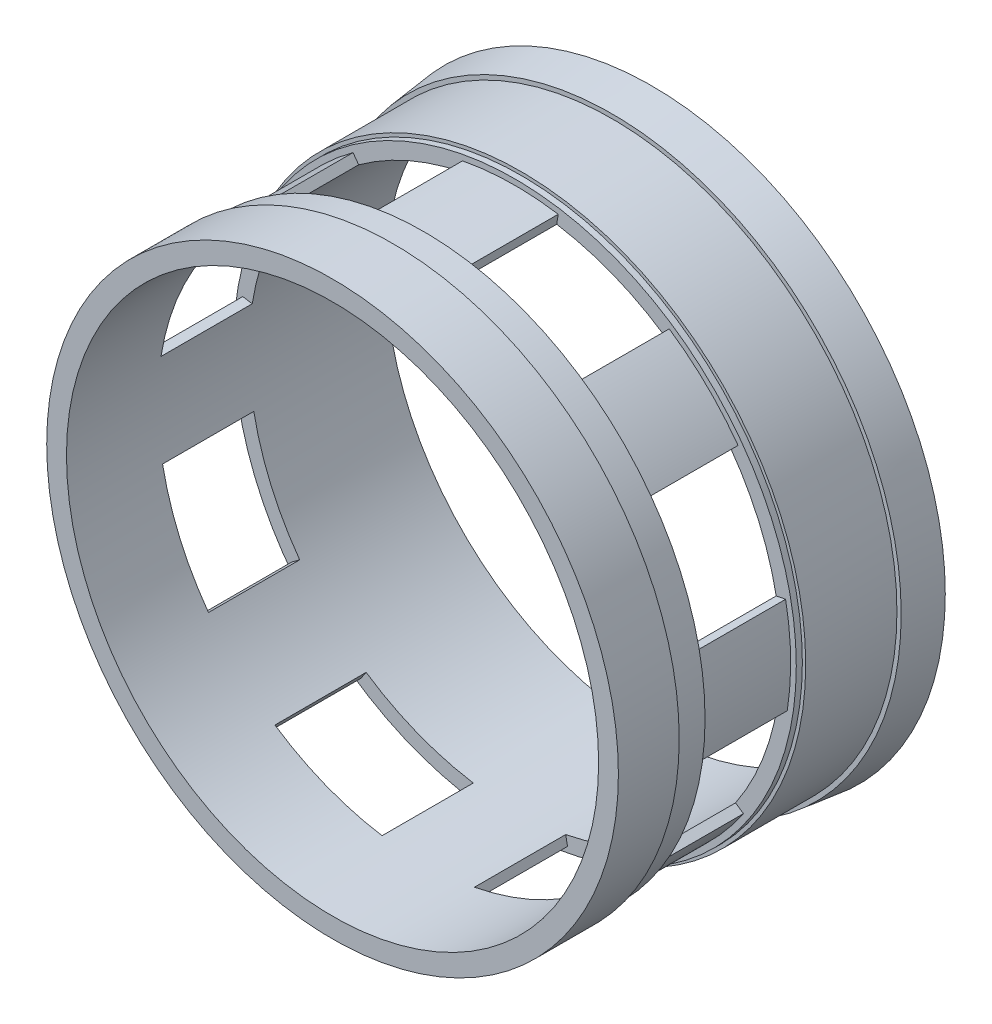
SolidWorks part; units mm, degrees
ref_plane "Front Plane" through (0, 0, 0) normal (0, 0, 1) x (1, 0, 0)
ref_plane "Top Plane" through (0, 0, 0) normal (0, 1, 0) x (1, 0, 0)
ref_plane "Right Plane" through (0, 0, 0) normal (1, 0, 0) x (0, 0, -1)
sketch "Sketch1" plane through (0, 0, 0) normal (0, 0, 1) x (1, 0, 0)
  circle A0 centre (0, 0) radius 9.65
  dimension "D1" = 19.3
ref_plane "Plane1" through (0, 0, 1.3) normal (0, 0, 1) x (1, 0, 0)
sketch "Sketch2" plane through (0, 0, 1.3) normal (0, 0, 1) x (1, 0, 0)
  circle A0 centre (0, 0) radius 9.5
  dimension "D1" = 19
loft "Loft2" add profiles "Sketch1", "Sketch2"
sketch "Sketch3" plane through (0, 0, 1.3) normal (0, 0, 1) x (1, 0, 0)
  circle A0 centre (0, 0) radius 9.36
  dimension "D1" = 18.72
extrude "Boss-Extrude1" add sketch "Sketch3" along normal blind 3
sketch "Sketch4" plane through (0, 0, 4.3) normal (0, 0, 1) x (1, 0, 0)
  circle A0 centre (0, 0) radius 9.25
  dimension "D1" = 18.5
extrude "Boss-Extrude2" add sketch "Sketch4" along normal blind 0.2
sketch "Sketch5" plane through (0, 0, 4.5) normal (0, 0, 1) x (1, 0, 0)
  circle A0 centre (0, 0) radius 8.75
  dimension "D1" = 17.5
extrude "Cut-Extrude1" cut sketch "Sketch5" against normal blind 10.2
sketch "Sketch7" plane through (0, 0, 4.5) normal (0, 0, 1) x (1, 0, 0)
  line L0 (-1.6668, 8.5898) -> (-1.7268, 8.8989)
  line L1 (0, 0) -> (-0.1765, 10.3009) construction
  line L2 (1.3716, 8.6418) -> (1.4209, 8.9528)
  arc A0 (1.3716, 8.6418) -> (-1.6668, 8.5898) centre (0, 0) ccw
  arc A1 (1.4209, 8.9528) -> (-1.7268, 8.8989) centre (0, 0) ccw
  dimension "D1" = 10
extrude "Boss-Extrude3" add sketch "Sketch7" along normal blind 3
pattern_circular "CirPattern1" count 8 over 360 about axis through (0, 0, 0) along (0, 0, 1) of "Boss-Extrude3"
sketch "Sketch8" plane through (0, 0, 7.5) normal (0, 0, 1) x (1, 0, 0)
  circle A0 centre (0, 0) radius 9.25
extrude "Boss-Extrude4" add sketch "Sketch8" along normal blind 1
sketch "Sketch9" plane through (0, 0, 8.5) normal (0, 0, 1) x (1, 0, 0)
  circle A0 centre (0, 0) radius 9.4
  dimension "D1" = 18.8
extrude "Boss-Extrude5" add sketch "Sketch9" along normal blind 2
sketch "Sketch11" plane through (0, 0, 10.5) normal (0, 0, 1) x (1, 0, 0)
  circle A0 centre (0, 0) radius 8.75
  dimension "D1" = 17.5
extrude "Cut-Extrude2" cut sketch "Sketch11" against normal blind 9
